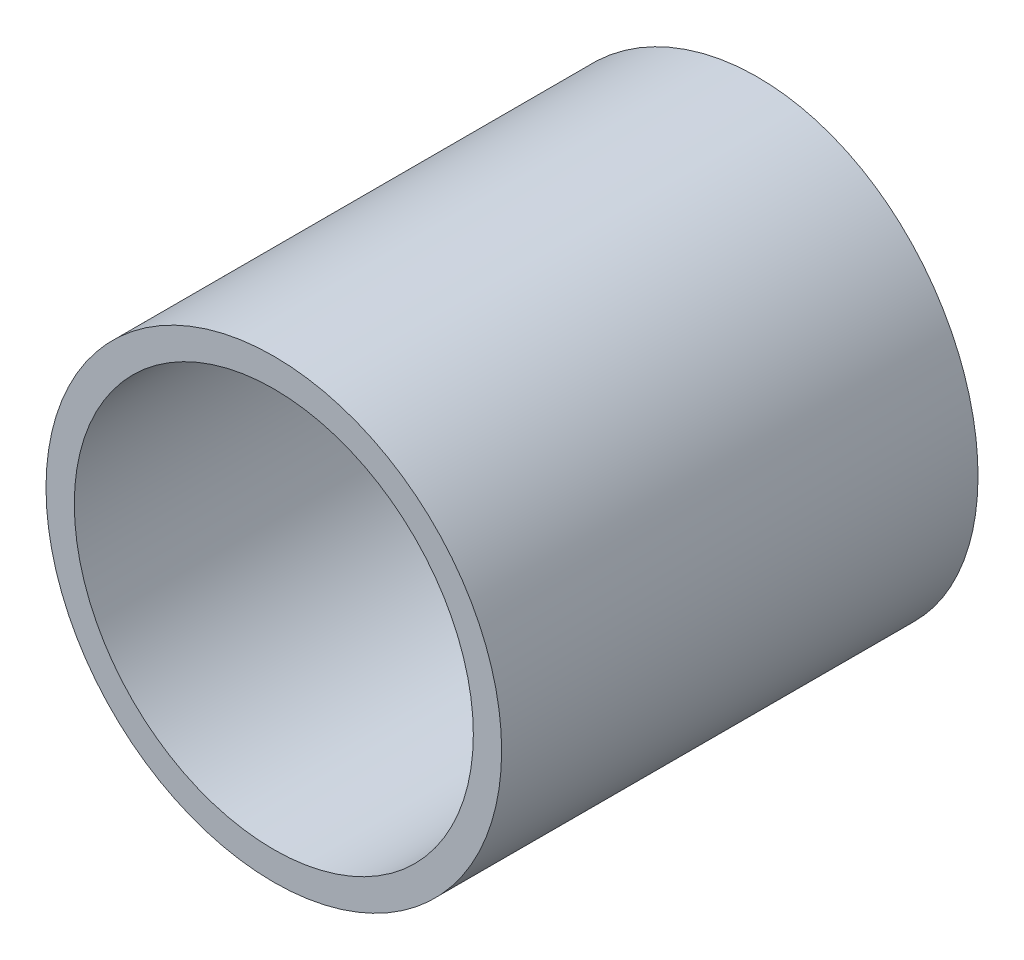
from build123d import *

# Parameters (mm, degrees)
SKETCH1_R           = 24.15
SKETCH1_R_2         = 21.15
BOSS_EXTRUDE1_DEPTH = 100
SKETCH3_R           = 379.5
CUT_EXTRUDE2_DEPTH  = 50


with BuildPart() as part:
    # Sketch1 → Boss-Extrude1 (new body)
    with BuildSketch(Plane.XY):
        Circle(SKETCH1_R)
        Circle(SKETCH1_R_2, mode=Mode.SUBTRACT)
    extrude(amount=BOSS_EXTRUDE1_DEPTH)

    # Sketch3 → Cut-Extrude2 (cut, symmetric)
    with BuildSketch(Plane(origin=(0, 0, 0), x_dir=(0, 0, -1), z_dir=(1, 0, 0))):
        with Locations((330, 0)):
            Circle(SKETCH3_R)
    extrude(amount=CUT_EXTRUDE2_DEPTH, both=True, mode=Mode.SUBTRACT)


solid = part.part
